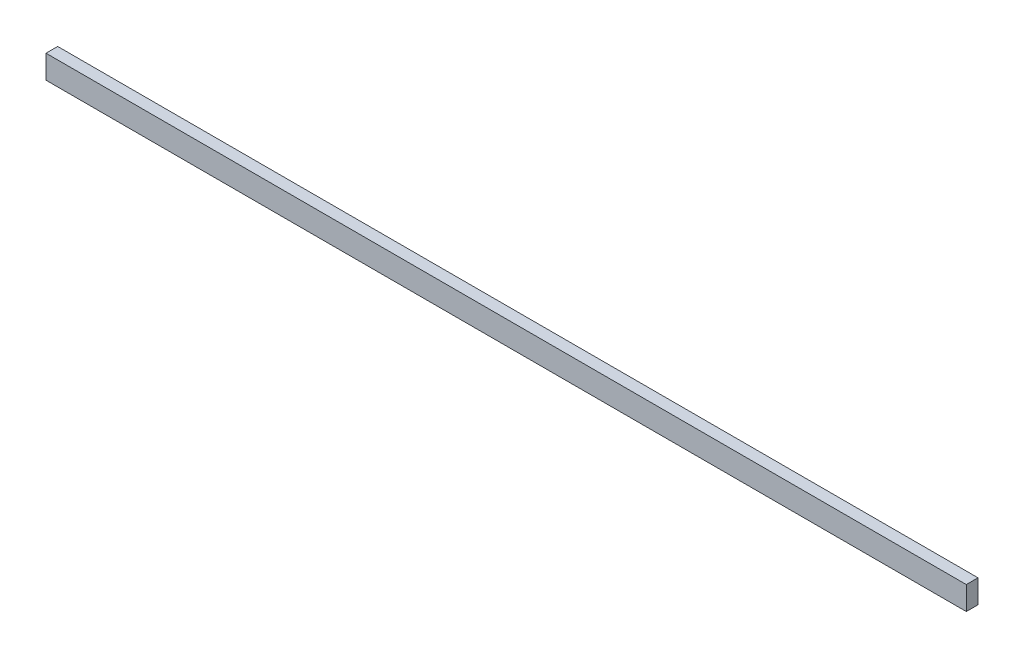
SolidWorks part; units mm, degrees
material "A3"
ref_plane "前视基准面" through (0, 0, 0) normal (0, 0, 1) x (1, 0, 0)
ref_plane "上视基准面" through (0, 0, 0) normal (0, 1, 0) x (1, 0, 0)
ref_plane "右视基准面" through (0, 0, 0) normal (1, 0, 0) x (0, 0, -1)
sketch "草图1" plane through (0, 0, 0) normal (0, 1, 0) x (1, 0, 0)
  line L1 (-590, -7.5) -> (590, -7.5)
  line L2 (-590, -7.5) -> (-590, 7.5)
  line L3 (-590, 7.5) -> (590, 7.5)
  line L4 (590, -7.5) -> (590, 7.5)
  line L5 (-590, -7.5) -> (590, 7.5) construction
  line L6 (-590, 7.5) -> (590, -7.5) construction
  point P0 (0, 0)
  dimension "D1" = 15
  dimension "D2" = 1180
extrude "凸台-拉伸1" add sketch "草图1" along normal mid plane 30
